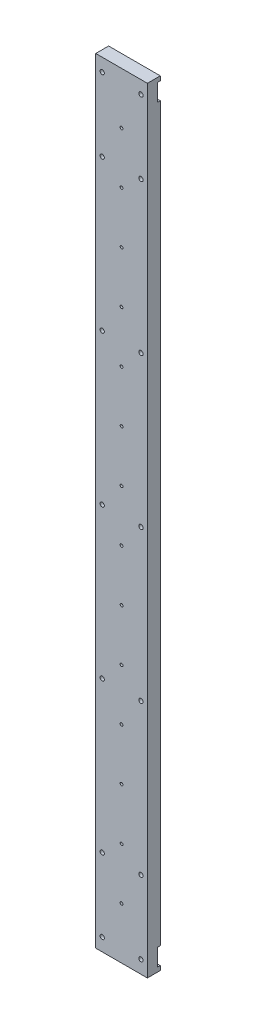
from build123d import *

# Parameters (mm, degrees)
SKETCH1_W           = 60
SKETCH1_H           = 900
BOSS_EXTRUDE1_DEPTH = 15
SKETCH5_W           = 60
SKETCH5_H           = 20
CUT_EXTRUDE2_DEPTH  = 3
SKETCH7_W           = 15
SKETCH7_H           = 850
CUT_EXTRUDE3_DEPTH  = 2
M4_TAPPED_HOLE1_D   = 3.3
LPATTERN1_COUNT     = 14
LPATTERN1_PITCH     = 60
M6_TAPPED_HOLE1_D   = 5
M6_TAPPED_HOLE2_D   = 5
LPATTERN2_COUNT     = 3
LPATTERN2_PITCH     = 175
LPATTERN2_COL_COUNT = 3
LPATTERN2_COL_PITCH = 175


with BuildPart() as part:
    # Sketch1 → Boss-Extrude1 (new body)
    with BuildSketch(Plane.XY):
        Rectangle(SKETCH1_W, SKETCH1_H)
    extrude(amount=BOSS_EXTRUDE1_DEPTH)

    # Sketch5 → Cut-Extrude2 (cut)
    with BuildSketch(Plane(origin=(0, 0, 0), x_dir=(-1, 0, 0), z_dir=(0, 0, -1))):
        with Locations((0, 435)):
            Rectangle(SKETCH5_W, SKETCH5_H)
        with Locations((0, -435)):
            Rectangle(SKETCH5_W, SKETCH5_H)
    extrude(amount=-CUT_EXTRUDE2_DEPTH, mode=Mode.SUBTRACT)

    # Sketch7 → Cut-Extrude3 (cut)
    with BuildSketch(Plane(origin=(0, 0, 0), x_dir=(-1, 0, 0), z_dir=(0, 0, -1))):
        Rectangle(SKETCH7_W, SKETCH7_H)
    extrude(amount=-CUT_EXTRUDE3_DEPTH, mode=Mode.SUBTRACT)

    # M4 Tapped Hole1 (through all)
    with Locations(Plane(origin=(0, 0, 2), x_dir=(-1, 0, 0), z_dir=(0, 0, -1))):
        with Locations((0, 390)):
            m4_tapped_hole1 = Hole(M4_TAPPED_HOLE1_D / 2)

    # LPattern1: M4 Tapped Hole1 ×14
    with Locations(*[(0, -i * LPATTERN1_PITCH, 0) for i in range(1, LPATTERN1_COUNT)]):
        add(m4_tapped_hole1, mode=Mode.SUBTRACT)

    # M6 Tapped Hole1 (through all)
    with Locations(Plane(origin=(0, 0, 3), x_dir=(-1, 0, 0), z_dir=(0, 0, -1))):
        with Locations((-22.5, 435), (22.5, 435), (-22.5, -435), (22.5, -435)):
            Hole(M6_TAPPED_HOLE1_D / 2)

    # M6 Tapped Hole2 (through all)
    with Locations(Plane.XY.offset(15)):
        with Locations((-22.5, 0), (22.5, 0)):
            m6_tapped_hole2 = Hole(M6_TAPPED_HOLE2_D / 2)

    # LPattern2: M6 Tapped Hole2 ×3
    with Locations(*[(0, -i * LPATTERN2_PITCH, 0) for i in range(1, LPATTERN2_COUNT)]):
        add(m6_tapped_hole2, mode=Mode.SUBTRACT)

    # LPattern2 col: M6 Tapped Hole2 ×3
    with Locations(*[(0, i * LPATTERN2_COL_PITCH, 0) for i in range(1, LPATTERN2_COL_COUNT)]):
        add(m6_tapped_hole2, mode=Mode.SUBTRACT)


solid = part.part
